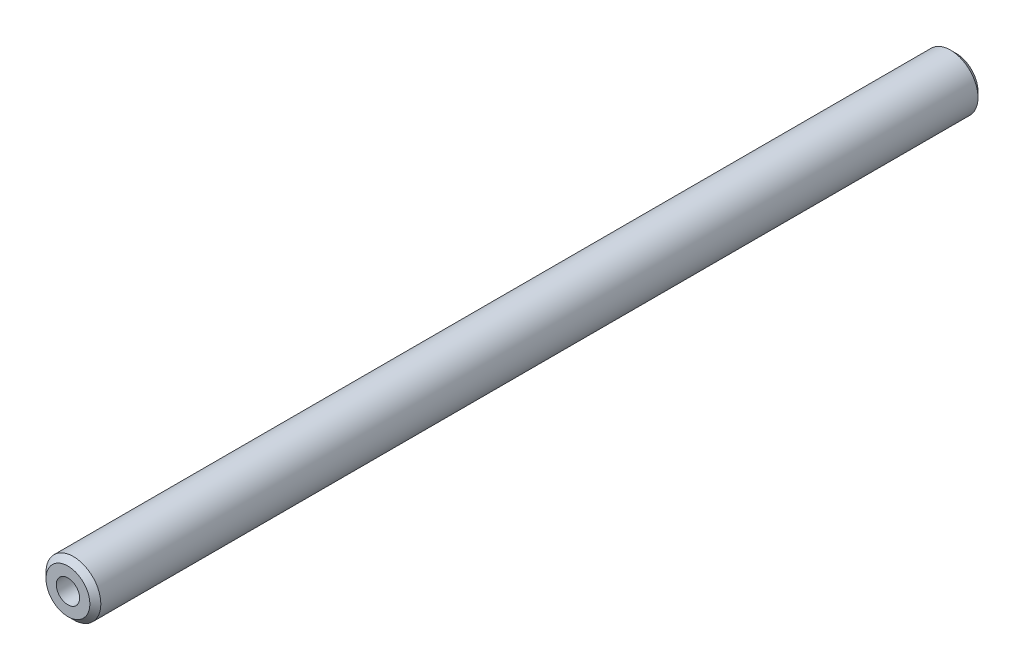
from build123d import *

# Parameters (mm, degrees)
SKETCH_1_R              = 10
EXTRUDE_1_DEPTH         = 162
CHAMFER_1_SIZE          = 2
HOLE_WIZARD_M10_1_D     = 8.5
HOLE_WIZARD_M10_1_DEPTH = 25
HOLE_WIZARD_M10_1_TIP   = 2.553657631
HOLE_WIZARD_M10_2_D     = 8.5
HOLE_WIZARD_M10_2_DEPTH = 25
HOLE_WIZARD_M10_2_TIP   = 2.553657631


with BuildPart() as part:
    # 草图1 → 凸台-拉伸1 (new, symmetric)
    with BuildSketch(Plane.XY):
        Circle(SKETCH_1_R)
    extrude(amount=EXTRUDE_1_DEPTH, both=True)

    # 倒角1
    chamfer_1_edges = [part.edges().sort_by_distance(p)[0] for p in [
        (-10, 0, -162),
        (-10, 0, 162),
    ]]
    chamfer(chamfer_1_edges, length=CHAMFER_1_SIZE)

    # M10 螺纹孔1
    with Locations(Plane.XY.offset(162)):
        with Locations((0, 0)):
            Hole(HOLE_WIZARD_M10_1_D / 2, depth=HOLE_WIZARD_M10_1_DEPTH)
            with Locations((0, 0, -(HOLE_WIZARD_M10_1_DEPTH + HOLE_WIZARD_M10_1_TIP / 2))):  # 118° drill point
                Cone(0, HOLE_WIZARD_M10_1_D / 2, HOLE_WIZARD_M10_1_TIP, mode=Mode.SUBTRACT)

    # M10 螺纹孔2
    with Locations(Plane(origin=(0, 0, -162), x_dir=(-1, 0, 0), z_dir=(0, 0, -1))):
        with Locations((0, 0)):
            Hole(HOLE_WIZARD_M10_2_D / 2, depth=HOLE_WIZARD_M10_2_DEPTH)
            with Locations((0, 0, -(HOLE_WIZARD_M10_2_DEPTH + HOLE_WIZARD_M10_2_TIP / 2))):  # 118° drill point
                Cone(0, HOLE_WIZARD_M10_2_D / 2, HOLE_WIZARD_M10_2_TIP, mode=Mode.SUBTRACT)


solid = part.part
